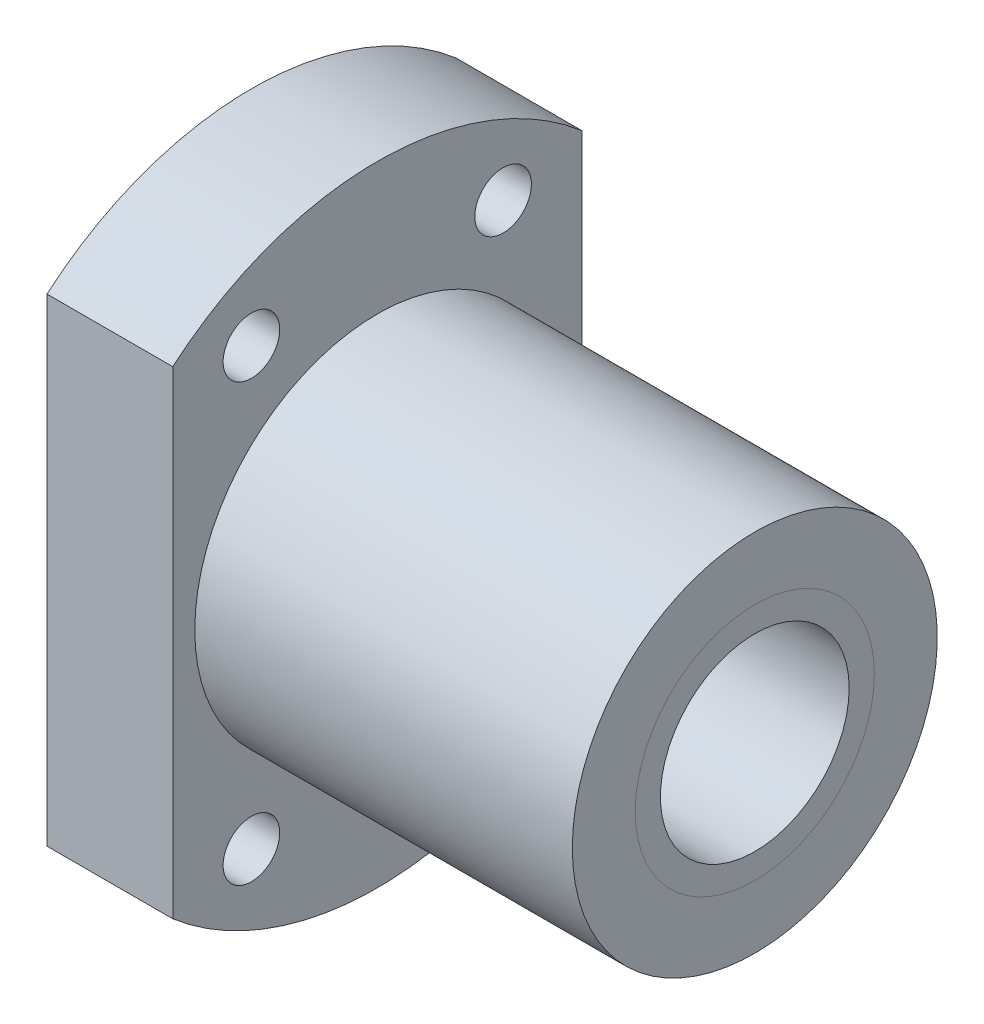
from build123d import *

# Parameters (mm, degrees)
HOLE_SIZE_PER_SOCKET_HEAD_CAP_SCREW_TYPE_D           = 9
HOLE_SIZE_PER_SOCKET_HEAD_CAP_SCREW_TYPE_CBORE_D     = 15
HOLE_SIZE_PER_SOCKET_HEAD_CAP_SCREW_TYPE_CBORE_DEPTH = 9
SKETCH4_OUTSIDE_W                                    = 134.496
SKETCH4_OUTSIDE_H                                    = 134.496
SKETCH4_OUTSIDE_W_2                                  = 65
SKETCH4_OUTSIDE_H_2                                  = 110
CUT_EXTRUDE1_DEPTH                                   = 107.77078252
SKETCH5_R                                            = 19
SKETCH5_R_2                                          = 15
BOSS_EXTRUDE1_DEPTH                                  = 40
SKETCH6_R                                            = 19
SKETCH6_R_2                                          = 15
BOSS_EXTRUDE2_DEPTH                                  = 40


with BuildPart() as part:
    # Sketch1 → Revolve1 (revolve)
    with BuildSketch(Plane.XY, mode=Mode.PRIVATE) as revolve1_sk:
        Polygon((0, 19), (0, 50), (20, 50), (20, 29), (80, 29), (80, 19), align=None)
    revolve(revolve1_sk.sketch.rotate(Axis((0, 0, 0), (1, 0, 0)), 90), axis=Axis((0, 0, 0), (1, 0, 0)))

    # Hole size per socket head cap screw type1 (through all)
    with Locations(Plane.ZY):
        with Locations((20, 34.641016151), (-20, 34.641016151), (-20, -34.641016151), (20, -34.641016151)):
            CounterBoreHole(HOLE_SIZE_PER_SOCKET_HEAD_CAP_SCREW_TYPE_D / 2, HOLE_SIZE_PER_SOCKET_HEAD_CAP_SCREW_TYPE_CBORE_D / 2, HOLE_SIZE_PER_SOCKET_HEAD_CAP_SCREW_TYPE_CBORE_DEPTH)

    # Sketch4 outside → Cut-Extrude1 (cut, through all)
    with BuildSketch(Plane.ZY):
        Rectangle(SKETCH4_OUTSIDE_W, SKETCH4_OUTSIDE_H)
        Rectangle(SKETCH4_OUTSIDE_W_2, SKETCH4_OUTSIDE_H_2, mode=Mode.SUBTRACT)
    extrude(amount=-CUT_EXTRUDE1_DEPTH, mode=Mode.SUBTRACT)


with BuildPart() as body_2:
    # Sketch5 → Boss-Extrude1 (new body)
    with BuildSketch(Plane(origin=(80, 0, 0), x_dir=(0, 0, -1), z_dir=(1, 0, 0))):
        Circle(SKETCH5_R)
        Circle(SKETCH5_R_2, mode=Mode.SUBTRACT)
    extrude(amount=-BOSS_EXTRUDE1_DEPTH)


with BuildPart() as body_3:
    # Sketch6 → Boss-Extrude2 (new body)
    with BuildSketch(Plane.ZY):
        Circle(SKETCH6_R)
        Circle(SKETCH6_R_2, mode=Mode.SUBTRACT)
    extrude(amount=-BOSS_EXTRUDE2_DEPTH)


solid = Compound([part.part, body_2.part, body_3.part])
